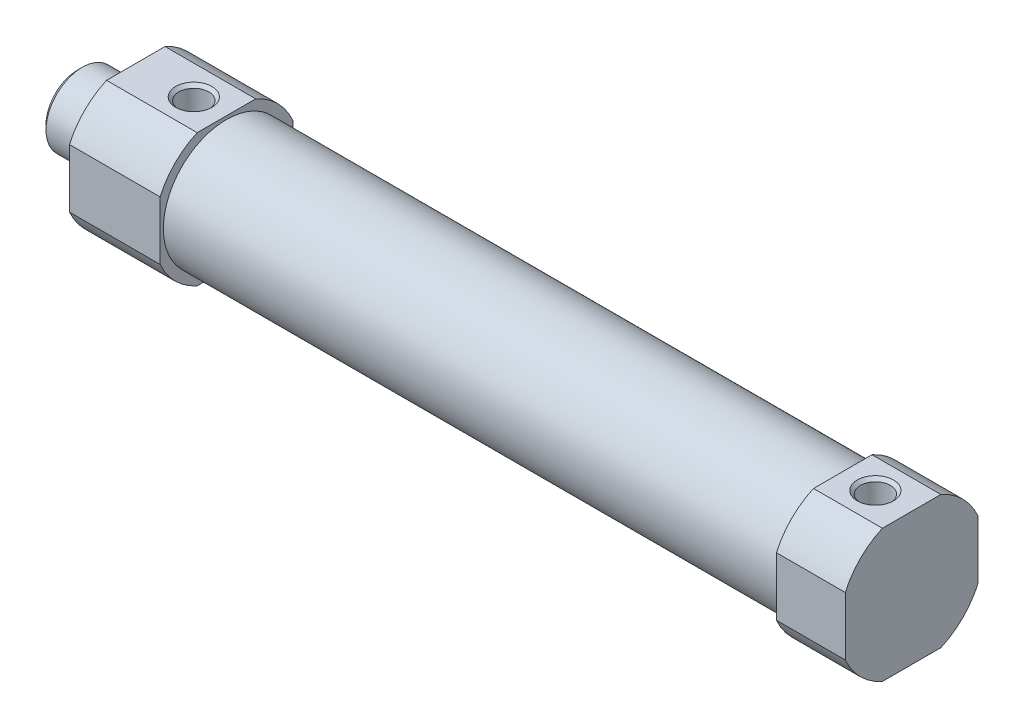
from build123d import *

# Parameters (mm, degrees)
EXTRUDE_1_DEPTH = 12.5
SKETCH_3_R      = 8.7
EXTRUDE_2_DEPTH = 85
EXTRUDE_3_DEPTH = 9.5


with BuildPart() as part:
    # 草图1 → 旋转1 (revolve)
    with BuildSketch(Plane.XY, mode=Mode.PRIVATE) as revolve_1_sk:
        Polygon((-8, 0), (-8, 4.3865), (-7.3865, 5), (0, 5), (0, 0), align=None)
    revolve(revolve_1_sk.sketch.rotate(Axis((0, 0, 0), (-1, 0, 0)), 270), axis=Axis((0, 0, 0), (-1, 0, 0)))

    # 草图2 → 凸台-拉伸1 (add)
    with BuildSketch(Plane(origin=(0, 0, 0), x_dir=(0, 0, -1), z_dir=(1, 0, 0))):
        with BuildLine():
            Line((-4.034538387, -9.15), (4.034538387, -9.15))
            ThreePointArc((4.034538387, -9.15), (7.071067812, -7.071067812), (9.15, -4.034538387))
            Line((9.15, -4.034538387), (9.15, 4.034538387))
            ThreePointArc((9.15, 4.034538387), (7.071067812, 7.071067812), (4.034538387, 9.15))
            Line((4.034538387, 9.15), (-4.034538387, 9.15))
            ThreePointArc((-4.034538387, 9.15), (-7.071067812, 7.071067812), (-9.15, 4.034538387))
            Line((-9.15, 4.034538387), (-9.15, -4.034538387))
            ThreePointArc((-9.15, -4.034538387), (-7.071067812, -7.071067812), (-4.034538387, -9.15))
        make_face()
    extrude(amount=EXTRUDE_1_DEPTH)

    # 草图3 → 凸台-拉伸2 (add)
    with BuildSketch(Plane(origin=(12.5, 0, 0), x_dir=(0, 0, -1), z_dir=(1, 0, 0))):
        Circle(SKETCH_3_R)
    extrude(amount=EXTRUDE_2_DEPTH)

    # 草图4 → 凸台-拉伸3 (add)
    with BuildSketch(Plane(origin=(97.5, 0, 0), x_dir=(0, 0, -1), z_dir=(1, 0, 0))):
        with BuildLine():
            Line((-4.034538387, -9.15), (4.034538387, -9.15))
            ThreePointArc((4.034538387, -9.15), (7.071067812, -7.071067812), (9.15, -4.034538387))
            Line((9.15, -4.034538387), (9.15, 4.034538387))
            ThreePointArc((9.15, 4.034538387), (7.071067812, 7.071067812), (4.034538387, 9.15))
            Line((4.034538387, 9.15), (-4.034538387, 9.15))
            ThreePointArc((-4.034538387, 9.15), (-7.071067812, 7.071067812), (-9.15, 4.034538387))
            Line((-9.15, 4.034538387), (-9.15, -4.034538387))
            ThreePointArc((-9.15, -4.034538387), (-7.071067812, -7.071067812), (-4.034538387, -9.15))
        make_face()
    extrude(amount=EXTRUDE_3_DEPTH)

    # 草图5 → 切除-旋转1 (revolve, cut)
    with BuildSketch(Plane.XY, mode=Mode.PRIVATE) as cut_revolve_1_sk:
        Polygon((8, 2.456616994), (5.933, 3.65), (5.933, 8.717), (5.5, 9.15), (8, 9.15), align=None)
    revolve(cut_revolve_1_sk.sketch.rotate(Axis((8, 9.15, 0), (0, -1, 0)), 90), axis=Axis((8, 9.15, 0), (0, -1, 0)), mode=Mode.SUBTRACT)

    # 草图6 → 切除-旋转2 (revolve, cut)
    with BuildSketch(Plane.XY, mode=Mode.PRIVATE) as cut_revolve_2_sk:
        Polygon((102, 2.456616994), (99.933, 3.65), (99.933, 8.717), (99.5, 9.15), (102, 9.15), align=None)
    revolve(cut_revolve_2_sk.sketch.rotate(Axis((102, 9.15, 0), (0, -1, 0)), 90), axis=Axis((102, 9.15, 0), (0, -1, 0)), mode=Mode.SUBTRACT)

    # 草图7 → 切除-旋转3 (revolve, cut)
    with BuildSketch(Plane.XY, mode=Mode.PRIVATE) as cut_revolve_3_sk:
        Polygon((-8, 0), (-8, 2.5), (12.5, 2.5), (12.5, 8), (77.5, 8), (77.5, 0), align=None)
    revolve(cut_revolve_3_sk.sketch.rotate(Axis((50, 0, 0), (-1, 0, 0)), 270), axis=Axis((50, 0, 0), (-1, 0, 0)), mode=Mode.SUBTRACT)


solid = part.part
